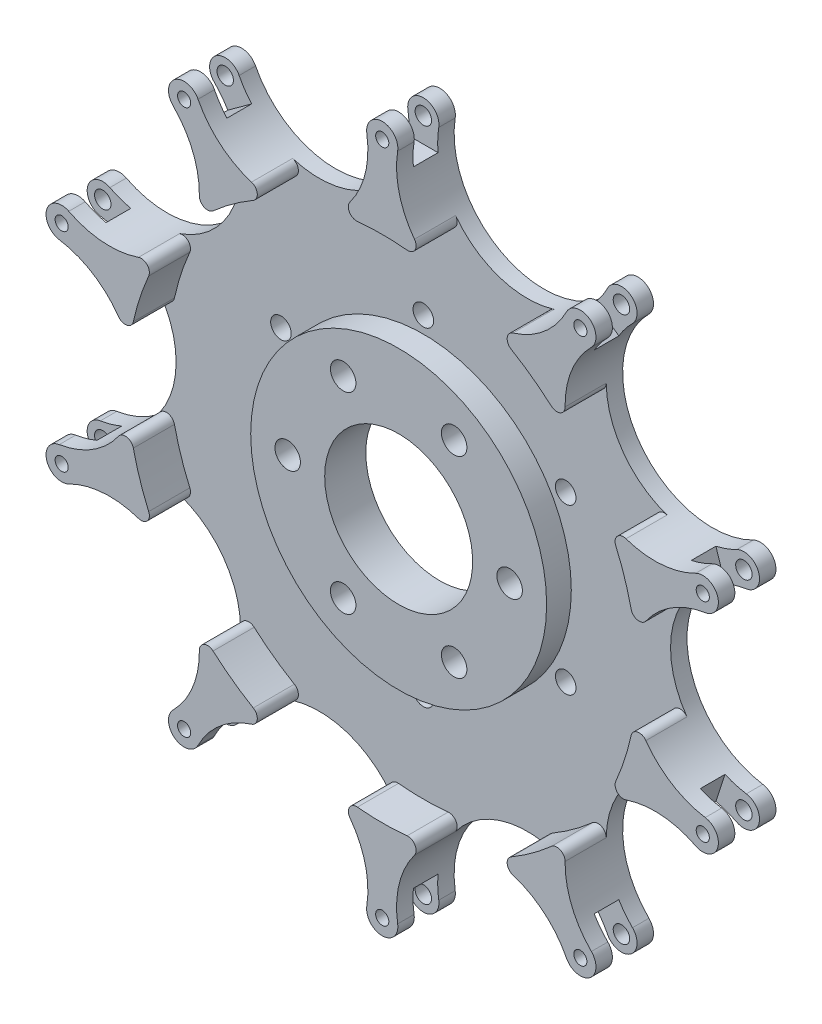
SolidWorks part; units mm, degrees
material "6061 合金"
ref_plane "前视基准面" through (0, 0, 0) normal (0, 0, 1) x (1, 0, 0)
ref_plane "上视基准面" through (0, 0, 0) normal (0, 1, 0) x (1, 0, 0)
ref_plane "右视基准面" through (0, 0, 0) normal (1, 0, 0) x (0, 0, -1)
sketch "草图1" plane through (0, 0, 0) normal (0, 0, 1) x (1, 0, 0)
  line L0 (0, 0) -> (0, 41) construction
  circle A0 centre (0, 0) radius 30.0724 construction
  circle A1 centre (0, 0) radius 41 construction
  arc A2 (1.8766, 40.7028) -> (-1.8766, 40.7028) centre (0, 41) ccw
  circle A3 centre (0, 41) radius 1
  arc A4 (1.8766, 40.7028) -> (9.2929, 28.6005) centre (12.6697, 38.9933) ccw
  arc A5 (-1.8766, 40.7028) -> (-9.2929, 28.6005) centre (-12.6697, 38.9933) cw
  circle A6 centre (0, 41) radius 2.5 construction
  arc A7 (25.4427, 31.8262) -> (24.3291, 17.6761) centre (33.1697, 24.0992) ccw
  arc A8 (22.4063, 34.0323) -> (9.2929, 28.6005) centre (12.6697, 38.9933) cw
  arc A9 (25.4427, 31.8262) -> (22.4063, 34.0323) centre (24.0992, 33.1697) ccw
  arc A10 (39.2905, 10.7931) -> (30.0724, 0) centre (41, 0) ccw
  arc A11 (38.1307, 14.3626) -> (24.3291, 17.6761) centre (33.1697, 24.0992) cw
  arc A12 (39.2905, 10.7931) -> (38.1307, 14.3626) centre (38.9933, 12.6697) ccw
  arc A13 (38.1307, -14.3626) -> (24.3291, -17.6761) centre (33.1697, -24.0992) ccw
  arc A14 (39.2905, -10.7931) -> (30.0724, 0) centre (41, 0) cw
  arc A15 (38.1307, -14.3626) -> (39.2905, -10.7931) centre (38.9933, -12.6697) ccw
  arc A16 (22.4063, -34.0323) -> (9.2929, -28.6005) centre (12.6697, -38.9933) ccw
  arc A17 (25.4427, -31.8262) -> (24.3291, -17.6761) centre (33.1697, -24.0992) cw
  arc A18 (22.4063, -34.0323) -> (25.4427, -31.8262) centre (24.0992, -33.1697) ccw
  arc A19 (-1.8766, -40.7028) -> (-9.2929, -28.6005) centre (-12.6697, -38.9933) ccw
  arc A20 (1.8766, -40.7028) -> (9.2929, -28.6005) centre (12.6697, -38.9933) cw
  arc A21 (-1.8766, -40.7028) -> (1.8766, -40.7028) centre (0, -41) ccw
  arc A22 (-25.4427, -31.8262) -> (-24.3291, -17.6761) centre (-33.1697, -24.0992) ccw
  arc A23 (-22.4063, -34.0323) -> (-9.2929, -28.6005) centre (-12.6697, -38.9933) cw
  arc A24 (-25.4427, -31.8262) -> (-22.4063, -34.0323) centre (-24.0992, -33.1697) ccw
  arc A25 (-39.2905, -10.7931) -> (-30.0724, 0) centre (-41, 0) ccw
  arc A26 (-38.1307, -14.3626) -> (-24.3291, -17.6761) centre (-33.1697, -24.0992) cw
  arc A27 (-39.2905, -10.7931) -> (-38.1307, -14.3626) centre (-38.9933, -12.6697) ccw
  arc A28 (-38.1307, 14.3626) -> (-24.3291, 17.6761) centre (-33.1697, 24.0992) ccw
  arc A29 (-39.2905, 10.7931) -> (-30.0724, 0) centre (-41, 0) cw
  arc A30 (-38.1307, 14.3626) -> (-39.2905, 10.7931) centre (-38.9933, 12.6697) ccw
  arc A31 (-22.4063, 34.0323) -> (-9.2929, 28.6005) centre (-12.6697, 38.9933) ccw
  arc A32 (-25.4427, 31.8262) -> (-24.3291, 17.6761) centre (-33.1697, 24.0992) cw
  arc A33 (-22.4063, 34.0323) -> (-25.4427, 31.8262) centre (-24.0992, 33.1697) ccw
  circle A34 centre (-12.6697, 38.9933) radius 9 construction
  circle A36 centre (24.0992, 33.1697) radius 1
  circle A37 centre (38.9933, 12.6697) radius 1
  circle A38 centre (38.9933, -12.6697) radius 1
  circle A39 centre (24.0992, -33.1697) radius 1
  circle A40 centre (0, -41) radius 1
  circle A41 centre (-24.0992, -33.1697) radius 1
  circle A42 centre (-38.9933, -12.6697) radius 1
  circle A43 centre (-38.9933, 12.6697) radius 1
  circle A44 centre (-24.0992, 33.1697) radius 1
  point P78 (0, 0)
  point P88 (0, 0)
  point P98 (0, 0)
  point P107 (0, 0)
  dimension "D1" = 10.9276
  dimension "D2" = 82
  dimension "D3" = 3.8
  dimension "D4" = 2
  dimension "D5" = 5
  dimension "D7" = 60.1447
  dimension "D8" = 18
  dimension "D6" = 10
  dimension "D9" = 10
extrude "外型" add sketch "草图1" along normal blind 2
sketch "草图4" plane through (0, 0, 0) normal (0, 0, -1) x (-1, 0, 0)
  circle A10 centre (0, 0) radius 20 construction
  point P2 (0, 20)
  point P5 (17.3205, 10)
  point P6 (17.3205, -10)
  point P7 (0, -20)
  point P8 (-17.3205, -10)
  point P10 (0, 0)
  point P27 (-17.3205, 10)
  dimension "D2" = 6
  dimension "D1" = 40
sketch "草图6" [suppressed] plane through (0, 0, 0) normal (0, 0, -1) x (-1, 0, 0)
  arc A20 (1.8766, 40.7028) -> (22.4063, 34.0323) centre (12.6697, 38.9933) ccw
  arc A21 (1.8766, 40.7028) -> (-1.8766, 40.7028) centre (0, 41) ccw
  arc A22 (-22.4063, 34.0323) -> (-1.8766, 40.7028) centre (-12.6697, 38.9933) ccw
  arc A23 (-22.4063, 34.0323) -> (-25.4427, 31.8262) centre (-24.0992, 33.1697) ccw
  arc A24 (-38.1307, 14.3626) -> (-25.4427, 31.8262) centre (-33.1697, 24.0992) ccw
  arc A25 (-38.1307, 14.3626) -> (-39.2905, 10.7931) centre (-38.9933, 12.6697) ccw
  arc A26 (-39.2905, -10.7931) -> (-39.2905, 10.7931) centre (-41, 0) ccw
  arc A27 (-39.2905, -10.7931) -> (-38.1307, -14.3626) centre (-38.9933, -12.6697) ccw
  arc A28 (-25.4427, -31.8262) -> (-38.1307, -14.3626) centre (-33.1697, -24.0992) ccw
  arc A29 (-25.4427, -31.8262) -> (-22.4063, -34.0323) centre (-24.0992, -33.1697) ccw
  arc A30 (-1.8766, -40.7028) -> (-22.4063, -34.0323) centre (-12.6697, -38.9933) ccw
  arc A31 (-1.8766, -40.7028) -> (1.8766, -40.7028) centre (0, -41) ccw
  arc A32 (22.4063, -34.0323) -> (1.8766, -40.7028) centre (12.6697, -38.9933) ccw
  arc A33 (22.4063, -34.0323) -> (25.4427, -31.8262) centre (24.0992, -33.1697) ccw
  arc A34 (38.1307, -14.3626) -> (25.4427, -31.8262) centre (33.1697, -24.0992) ccw
  arc A35 (38.1307, -14.3626) -> (39.2905, -10.7931) centre (38.9933, -12.6697) ccw
  arc A36 (39.2905, 10.7931) -> (39.2905, -10.7931) centre (41, 0) ccw
  arc A37 (39.2905, 10.7931) -> (38.1307, 14.3626) centre (38.9933, 12.6697) ccw
  arc A38 (25.4427, 31.8262) -> (38.1307, 14.3626) centre (33.1697, 24.0992) ccw
  arc A39 (25.4427, 31.8262) -> (22.4063, 34.0323) centre (24.0992, 33.1697) ccw
  arc A40 (1.8766, 40.7028) -> (22.4063, 34.0323) centre (12.6697, 38.9933) ccw
  arc A41 (1.8766, 40.7028) -> (-1.8766, 40.7028) centre (0, 41) ccw
  arc A42 (-22.4063, 34.0323) -> (-1.8766, 40.7028) centre (-12.6697, 38.9933) ccw
  arc A43 (-22.4063, 34.0323) -> (-25.4427, 31.8262) centre (-24.0992, 33.1697) ccw
  arc A44 (-38.1307, 14.3626) -> (-25.4427, 31.8262) centre (-33.1697, 24.0992) ccw
  arc A45 (-38.1307, 14.3626) -> (-39.2905, 10.7931) centre (-38.9933, 12.6697) ccw
  arc A46 (-39.2905, -10.7931) -> (-39.2905, 10.7931) centre (-41, 0) ccw
  arc A47 (-39.2905, -10.7931) -> (-38.1307, -14.3626) centre (-38.9933, -12.6697) ccw
  arc A48 (-25.4427, -31.8262) -> (-38.1307, -14.3626) centre (-33.1697, -24.0992) ccw
  arc A49 (-25.4427, -31.8262) -> (-22.4063, -34.0323) centre (-24.0992, -33.1697) ccw
  arc A50 (-1.8766, -40.7028) -> (-22.4063, -34.0323) centre (-12.6697, -38.9933) ccw
  arc A51 (-1.8766, -40.7028) -> (1.8766, -40.7028) centre (0, -41) ccw
  arc A52 (22.4063, -34.0323) -> (1.8766, -40.7028) centre (12.6697, -38.9933) ccw
  arc A53 (22.4063, -34.0323) -> (25.4427, -31.8262) centre (24.0992, -33.1697) ccw
  arc A54 (38.1307, -14.3626) -> (25.4427, -31.8262) centre (33.1697, -24.0992) ccw
  arc A55 (38.1307, -14.3626) -> (39.2905, -10.7931) centre (38.9933, -12.6697) ccw
  arc A56 (39.2905, 10.7931) -> (39.2905, -10.7931) centre (41, 0) ccw
  arc A57 (39.2905, 10.7931) -> (38.1307, 14.3626) centre (38.9933, 12.6697) ccw
  arc A58 (25.4427, 31.8262) -> (38.1307, 14.3626) centre (33.1697, 24.0992) ccw
  arc A59 (25.4427, 31.8262) -> (22.4063, 34.0323) centre (24.0992, 33.1697) ccw
  dimension "D1" = 0
extrude "切除-拉伸3" [suppressed] cut sketch "草图6" against normal up to next
sketch "草图7" plane through (0, 0, 0) normal (0, 0, -1) x (-1, 0, 0)
  line L0 (0, 0) -> (13.5, 0) construction
  circle A0 centre (0, 0) radius 13.5 construction
  circle A1 centre (13.5, 0) radius 1.55
  circle A2 centre (6.75, -11.6913) radius 1.55
  circle A3 centre (0, 0) radius 13.5 construction
  circle A4 centre (-6.75, -11.6913) radius 1.55
  circle A5 centre (0, 0) radius 13.5 construction
  circle A6 centre (-13.5, 0) radius 1.55
  circle A7 centre (0, 0) radius 13.5 construction
  circle A8 centre (-6.75, 11.6913) radius 1.55
  circle A9 centre (0, 0) radius 13.5 construction
  circle A10 centre (6.75, 11.6913) radius 1.55
  circle A11 centre (0, 0) radius 13.5 construction
  circle A12 centre (0, 0) radius 9
  circle A13 centre (0, 13.5) radius 2 construction
  circle A14 centre (11.6913, 6.75) radius 2 construction
  circle A15 centre (11.6913, -6.75) radius 2 construction
  circle A16 centre (0, -13.5) radius 2 construction
  circle A17 centre (-11.6913, -6.75) radius 2 construction
  circle A18 centre (-11.6913, 6.75) radius 2 construction
  point P23 (0, 0)
  point P36 (0, 0)
  dimension "D1" = 27
  dimension "D2" = 3.1
  dimension "D4" = 18
  dimension "D5" = 4
  dimension "D3" = 6
  dimension "D6" = 6
hole_wizard "M3 螺纹孔1" positions "草图4" profile "草图15" tap size "M3" standard "GB" end condition through all
sketch "草图15" plane through (17.3205, 10, 0) normal (1, 0, 0) x (0, 1, 0)
  line L0 (0, 0) -> (0, 2)
  line L1 (0, 2) -> (1.25, 2)
  line L2 (1.25, 2) -> (1.25, 0)
  line L5 (1.25, 0) -> (0, 0)
  line L11 (0, -6.35) -> (0, 107.95) construction
  dimension "通孔螺纹孔钻头直径" = 2.5
  dimension "通孔螺纹孔钻头深度" = 2
cosmetic thread "孔螺纹线1" parameters "D2"=3
cosmetic thread "孔螺纹线3" parameters "D2"=3
cosmetic thread "孔螺纹线4" parameters "D2"=3
cosmetic thread "孔螺纹线5" parameters "D2"=3
cosmetic thread "孔螺纹线6" parameters "D2"=3
cosmetic thread "孔螺纹线7" parameters "D2"=3
cosmetic thread "孔螺纹线18" parameters "D2"=3
extrude "连接电机" cut sketch "草图7" against normal up to next
sketch "草图8" plane through (0, 0, 0) normal (0, 0, -1) x (-1, 0, 0)
  line L1 (-12.5, -20) -> (12.5, -20) construction
  line L2 (-12.5, -20) -> (-12.5, 20) construction
  line L3 (-12.5, 20) -> (12.5, 20) construction
  line L4 (12.5, -20) -> (12.5, 20) construction
  line L5 (-12.5, -20) -> (12.5, 20) construction
  line L6 (-12.5, 20) -> (12.5, -20) construction
  circle A0 centre (-12.5, 20) radius 3.1
  circle A1 centre (12.5, 20) radius 3.1
  circle A2 centre (12.5, -20) radius 3.1
  circle A3 centre (-12.5, -20) radius 3.1
  point P0 (0, 0)
  dimension "D3" = 6.2
  dimension "D1" = 40
  dimension "D2" = 25
extrude "预留孔位" [suppressed] cut sketch "草图8" against normal up to next
sketch "草图12" plane through (0, 0, 2) normal (0, 0, -1) x (-1, 0, 0)
  circle A0 centre (6.75, 11.6913) radius 1.55 construction
  circle A1 centre (13.5, 0) radius 1.55 construction
  circle A2 centre (6.75, -11.6913) radius 1.55 construction
  circle A3 centre (-6.75, -11.6913) radius 1.55 construction
  circle A4 centre (-13.5, 0) radius 1.55 construction
  circle A5 centre (-6.75, 11.6913) radius 1.55 construction
  circle A6 centre (0, 0) radius 9 construction
  circle A7 centre (6.75, 11.6913) radius 1.55
  circle A8 centre (13.5, 0) radius 1.55
  circle A9 centre (6.75, -11.6913) radius 1.55
  circle A10 centre (-6.75, -11.6913) radius 1.55
  circle A11 centre (-13.5, 0) radius 1.55
  circle A12 centre (-6.75, 11.6913) radius 1.55
  circle A13 centre (0, 0) radius 9
  circle A14 centre (0, 0) radius 18
  dimension "D1" = 36
extrude "凸台-拉伸1" add sketch "草图12" against normal blind 3
sketch "草图13" plane through (0, 0, 2) normal (0, 0, 1) x (1, 0, 0)
  line L0 (-1.7873, 38) -> (1.7873, 38)
  line L1 (20.8899, 31.7932) -> (23.7818, 29.6921)
  line L2 (35.5878, 13.4425) -> (36.6925, 10.0428)
  line L3 (36.6925, -10.0428) -> (35.5878, -13.4425)
  line L4 (23.7818, -29.6921) -> (20.8899, -31.7932)
  line L5 (1.7873, -38) -> (-1.7873, -38)
  line L6 (-20.8899, -31.7932) -> (-23.7818, -29.6921)
  line L7 (-35.5878, -13.4425) -> (-36.6925, -10.0428)
  line L8 (-36.6925, 10.0428) -> (-35.5878, 13.4425)
  line L9 (-23.7818, 29.6921) -> (-20.8899, 31.7932)
  circle A0 centre (0, 0) radius 30 construction
  arc A3 (-3.9202, 32.4467) -> (-1.7873, 38) centre (-12.6697, 38.9933) ccw
  arc A5 (3.022, 30.8524) -> (-3.022, 30.8524) centre (0, 0) ccw
  arc A6 (-3.022, 30.8524) -> (-3.9202, 32.4467) centre (-3.1195, 31.8476) cw
  arc A7 (3.9202, 32.4467) -> (3.022, 30.8524) centre (3.1195, 31.8476) cw
  circle A10 centre (0, 34.5) radius 1.5 construction
  arc A11 (-22.4063, 34.0323) -> (-1.8766, 40.7028) centre (-12.6697, 38.9933) ccw construction
  circle A20 centre (0, 41) radius 1 construction
  arc A21 (-22.4063, 34.0323) -> (-1.8766, 40.7028) centre (-12.6697, 38.9933) ccw
  arc A22 (-22.4063, 34.0323) -> (-25.4427, 31.8262) centre (-24.0992, 33.1697) ccw
  arc A23 (-38.1307, 14.3626) -> (-25.4427, 31.8262) centre (-33.1697, 24.0992) ccw
  arc A24 (-38.1307, 14.3626) -> (-39.2905, 10.7931) centre (-38.9933, 12.6697) ccw
  arc A25 (-39.2905, -10.7931) -> (-39.2905, 10.7931) centre (-41, 0) ccw
  arc A26 (-39.2905, -10.7931) -> (-38.1307, -14.3626) centre (-38.9933, -12.6697) ccw
  arc A27 (-25.4427, -31.8262) -> (-38.1307, -14.3626) centre (-33.1697, -24.0992) ccw
  arc A28 (-25.4427, -31.8262) -> (-22.4063, -34.0323) centre (-24.0992, -33.1697) ccw
  arc A29 (-1.8766, -40.7028) -> (-22.4063, -34.0323) centre (-12.6697, -38.9933) ccw
  arc A30 (-1.8766, -40.7028) -> (1.8766, -40.7028) centre (0, -41) ccw
  arc A31 (22.4063, -34.0323) -> (1.8766, -40.7028) centre (12.6697, -38.9933) ccw
  arc A32 (22.4063, -34.0323) -> (25.4427, -31.8262) centre (24.0992, -33.1697) ccw
  arc A33 (38.1307, -14.3626) -> (25.4427, -31.8262) centre (33.1697, -24.0992) ccw
  arc A34 (38.1307, -14.3626) -> (39.2905, -10.7931) centre (38.9933, -12.6697) ccw
  arc A35 (39.2905, 10.7931) -> (39.2905, -10.7931) centre (41, 0) ccw
  arc A36 (39.2905, 10.7931) -> (38.1307, 14.3626) centre (38.9933, 12.6697) ccw
  arc A37 (25.4427, 31.8262) -> (38.1307, 14.3626) centre (33.1697, 24.0992) ccw
  arc A38 (25.4427, 31.8262) -> (22.4063, 34.0323) centre (24.0992, 33.1697) ccw
  arc A39 (1.8766, 40.7028) -> (22.4063, 34.0323) centre (12.6697, 38.9933) ccw
  arc A40 (1.8766, 40.7028) -> (-1.8766, 40.7028) centre (0, 41) ccw
  arc A59 (1.7873, 38) -> (3.9202, 32.4467) centre (12.6697, 38.9933) ccw
  arc A68 (23.7818, 29.6921) -> (22.2431, 23.9457) centre (33.1697, 24.0992) ccw
  arc A77 (22.2431, 23.9457) -> (20.5794, 23.1838) centre (21.2432, 23.9317) cw
  arc A80 (20.5794, 23.1838) -> (15.6897, 26.7364) centre (0, 0) ccw
  arc A81 (15.6897, 26.7364) -> (15.9002, 28.5541) centre (16.1958, 27.5988) cw
  arc A82 (15.9002, 28.5541) -> (20.8899, 31.7932) centre (12.6697, 38.9933) ccw
  arc A83 (36.6925, 10.0428) -> (32.07, 6.2983) centre (41, 0) ccw
  arc A84 (32.07, 6.2983) -> (30.2762, 6.6598) centre (31.2528, 6.8747) cw
  arc A85 (30.2762, 6.6598) -> (28.4085, 12.408) centre (0, 0) ccw
  arc A86 (28.4085, 12.408) -> (29.6472, 13.7549) centre (29.3249, 12.8082) cw
  arc A87 (29.6472, 13.7549) -> (35.5878, 13.4425) centre (33.1697, 24.0992) ccw
  arc A88 (35.5878, -13.4425) -> (29.6472, -13.7549) centre (33.1697, -24.0992) ccw
  arc A89 (29.6472, -13.7549) -> (28.4085, -12.408) centre (29.3249, -12.8082) cw
  arc A90 (28.4085, -12.408) -> (30.2762, -6.6598) centre (0, 0) ccw
  arc A91 (30.2762, -6.6598) -> (32.07, -6.2983) centre (31.2528, -6.8747) cw
  arc A92 (32.07, -6.2983) -> (36.6925, -10.0428) centre (41, 0) ccw
  arc A93 (20.8899, -31.7932) -> (15.9002, -28.5541) centre (12.6697, -38.9933) ccw
  arc A94 (15.9002, -28.5541) -> (15.6897, -26.7364) centre (16.1958, -27.5988) cw
  arc A95 (15.6897, -26.7364) -> (20.5794, -23.1838) centre (0, 0) ccw
  arc A96 (20.5794, -23.1838) -> (22.2431, -23.9457) centre (21.2432, -23.9317) cw
  arc A97 (22.2431, -23.9457) -> (23.7818, -29.6921) centre (33.1697, -24.0992) ccw
  arc A98 (-1.7873, -38) -> (-3.9202, -32.4467) centre (-12.6697, -38.9933) ccw
  arc A99 (-3.9202, -32.4467) -> (-3.022, -30.8524) centre (-3.1195, -31.8476) cw
  arc A100 (-3.022, -30.8524) -> (3.022, -30.8524) centre (0, 0) ccw
  arc A101 (3.022, -30.8524) -> (3.9202, -32.4467) centre (3.1195, -31.8476) cw
  arc A102 (3.9202, -32.4467) -> (1.7873, -38) centre (12.6697, -38.9933) ccw
  arc A103 (-23.7818, -29.6921) -> (-22.2431, -23.9457) centre (-33.1697, -24.0992) ccw
  arc A104 (-22.2431, -23.9457) -> (-20.5794, -23.1838) centre (-21.2432, -23.9317) cw
  arc A105 (-20.5794, -23.1838) -> (-15.6897, -26.7364) centre (0, 0) ccw
  arc A106 (-15.6897, -26.7364) -> (-15.9002, -28.5541) centre (-16.1958, -27.5988) cw
  arc A107 (-15.9002, -28.5541) -> (-20.8899, -31.7932) centre (-12.6697, -38.9933) ccw
  arc A108 (-36.6925, -10.0428) -> (-32.07, -6.2983) centre (-41, 0) ccw
  arc A109 (-32.07, -6.2983) -> (-30.2762, -6.6598) centre (-31.2528, -6.8747) cw
  arc A110 (-30.2762, -6.6598) -> (-28.4085, -12.408) centre (0, 0) ccw
  arc A111 (-28.4085, -12.408) -> (-29.6472, -13.7549) centre (-29.3249, -12.8082) cw
  arc A112 (-29.6472, -13.7549) -> (-35.5878, -13.4425) centre (-33.1697, -24.0992) ccw
  arc A113 (-35.5878, 13.4425) -> (-29.6472, 13.7549) centre (-33.1697, 24.0992) ccw
  arc A114 (-29.6472, 13.7549) -> (-28.4085, 12.408) centre (-29.3249, 12.8082) cw
  arc A115 (-28.4085, 12.408) -> (-30.2762, 6.6598) centre (0, 0) ccw
  arc A116 (-30.2762, 6.6598) -> (-32.07, 6.2983) centre (-31.2528, 6.8747) cw
  arc A117 (-32.07, 6.2983) -> (-36.6925, 10.0428) centre (-41, 0) ccw
  arc A118 (-20.8899, 31.7932) -> (-15.9002, 28.5541) centre (-12.6697, 38.9933) ccw
  arc A119 (-15.9002, 28.5541) -> (-15.6897, 26.7364) centre (-16.1958, 27.5988) cw
  arc A120 (-15.6897, 26.7364) -> (-20.5794, 23.1838) centre (0, 0) ccw
  arc A121 (-20.5794, 23.1838) -> (-22.2431, 23.9457) centre (-21.2432, 23.9317) cw
  arc A122 (-22.2431, 23.9457) -> (-23.7818, 29.6921) centre (-33.1697, 24.0992) ccw
  point P27 (-5.8696, 30.4392)
  point P36 (5.8696, 30.4392)
  point P152 (0, 0)
  point P217 (0, 0)
  dimension "D1" = 60
  dimension "D3" = 3
  dimension "D4" = 10
  dimension "D5" = 1
  dimension "D6" = 1
  dimension "D7" = 3
  dimension "D8" = 6.5
  dimension "D2" = 0
extrude "凸台-拉伸2" add sketch "草图13" along normal blind 3
sketch "草图14" plane through (0, 0, 5) normal (0, 0, 1) x (1, 0, 0)
  arc A0 (1.8766, 40.7028) -> (1.7873, 38) centre (12.6697, 38.9933) ccw construction
  arc A1 (1.8766, 40.7028) -> (-1.8766, 40.7028) centre (0, 41) ccw construction
  arc A2 (-1.7873, 38) -> (-1.8766, 40.7028) centre (-12.6697, 38.9933) ccw construction
  arc A3 (-3.9202, 32.4467) -> (-3.022, 30.8524) centre (-3.1195, 31.8476) ccw construction
  arc A4 (3.022, 30.8524) -> (-3.022, 30.8524) centre (0, 0) ccw construction
  arc A5 (3.022, 30.8524) -> (3.9202, 32.4467) centre (3.1195, 31.8476) ccw construction
  arc A6 (1.7873, 38) -> (3.9202, 32.4467) centre (12.6697, 38.9933) ccw construction
  arc A7 (-3.9202, 32.4467) -> (-1.7873, 38) centre (-12.6697, 38.9933) ccw construction
  arc A8 (1.8766, 40.7028) -> (1.7873, 38) centre (12.6697, 38.9933) ccw
  arc A9 (1.8766, 40.7028) -> (-1.8766, 40.7028) centre (0, 41) ccw
  arc A10 (-1.7873, 38) -> (-1.8766, 40.7028) centre (-12.6697, 38.9933) ccw
  arc A11 (-3.9202, 32.4467) -> (-3.022, 30.8524) centre (-3.1195, 31.8476) ccw
  arc A12 (3.022, 30.8524) -> (-3.022, 30.8524) centre (0, 0) ccw
  arc A13 (3.022, 30.8524) -> (3.9202, 32.4467) centre (3.1195, 31.8476) ccw
  arc A14 (1.7873, 38) -> (3.9202, 32.4467) centre (12.6697, 38.9933) ccw
  arc A15 (-3.9202, 32.4467) -> (-1.7873, 38) centre (-12.6697, 38.9933) ccw
  arc A18 (20.8899, 31.7932) -> (22.4063, 34.0323) centre (12.6697, 38.9933) ccw
  arc A19 (25.4427, 31.8262) -> (22.4063, 34.0323) centre (24.0992, 33.1697) ccw
  arc A20 (25.4427, 31.8262) -> (23.7818, 29.6921) centre (33.1697, 24.0992) ccw
  arc A21 (23.7818, 29.6921) -> (22.2431, 23.9457) centre (33.1697, 24.0992) ccw
  arc A22 (20.5794, 23.1838) -> (22.2431, 23.9457) centre (21.2432, 23.9317) ccw
  arc A23 (20.5794, 23.1838) -> (15.6897, 26.7364) centre (0, 0) ccw
  arc A24 (15.9002, 28.5541) -> (15.6897, 26.7364) centre (16.1958, 27.5988) ccw
  arc A25 (15.9002, 28.5541) -> (20.8899, 31.7932) centre (12.6697, 38.9933) ccw
  arc A27 (35.5878, 13.4425) -> (38.1307, 14.3626) centre (33.1697, 24.0992) ccw
  arc A28 (39.2905, 10.7931) -> (38.1307, 14.3626) centre (38.9933, 12.6697) ccw
  arc A29 (39.2905, 10.7931) -> (36.6925, 10.0428) centre (41, 0) ccw
  arc A30 (36.6925, 10.0428) -> (32.07, 6.2983) centre (41, 0) ccw
  arc A31 (30.2762, 6.6598) -> (32.07, 6.2983) centre (31.2528, 6.8747) ccw
  arc A32 (30.2762, 6.6598) -> (28.4085, 12.408) centre (0, 0) ccw
  arc A33 (29.6472, 13.7549) -> (28.4085, 12.408) centre (29.3249, 12.8082) ccw
  arc A34 (29.6472, 13.7549) -> (35.5878, 13.4425) centre (33.1697, 24.0992) ccw
  arc A36 (36.6925, -10.0428) -> (39.2905, -10.7931) centre (41, 0) ccw
  arc A37 (38.1307, -14.3626) -> (39.2905, -10.7931) centre (38.9933, -12.6697) ccw
  arc A38 (38.1307, -14.3626) -> (35.5878, -13.4425) centre (33.1697, -24.0992) ccw
  arc A39 (35.5878, -13.4425) -> (29.6472, -13.7549) centre (33.1697, -24.0992) ccw
  arc A40 (28.4085, -12.408) -> (29.6472, -13.7549) centre (29.3249, -12.8082) ccw
  arc A41 (28.4085, -12.408) -> (30.2762, -6.6598) centre (0, 0) ccw
  arc A42 (32.07, -6.2983) -> (30.2762, -6.6598) centre (31.2528, -6.8747) ccw
  arc A43 (32.07, -6.2983) -> (36.6925, -10.0428) centre (41, 0) ccw
  arc A45 (23.7818, -29.6921) -> (25.4427, -31.8262) centre (33.1697, -24.0992) ccw
  arc A46 (22.4063, -34.0323) -> (25.4427, -31.8262) centre (24.0992, -33.1697) ccw
  arc A47 (22.4063, -34.0323) -> (20.8899, -31.7932) centre (12.6697, -38.9933) ccw
  arc A48 (20.8899, -31.7932) -> (15.9002, -28.5541) centre (12.6697, -38.9933) ccw
  arc A49 (15.6897, -26.7364) -> (15.9002, -28.5541) centre (16.1958, -27.5988) ccw
  arc A50 (15.6897, -26.7364) -> (20.5794, -23.1838) centre (0, 0) ccw
  arc A51 (22.2431, -23.9457) -> (20.5794, -23.1838) centre (21.2432, -23.9317) ccw
  arc A52 (22.2431, -23.9457) -> (23.7818, -29.6921) centre (33.1697, -24.0992) ccw
  arc A54 (1.7873, -38) -> (1.8766, -40.7028) centre (12.6697, -38.9933) ccw
  arc A55 (-1.8766, -40.7028) -> (1.8766, -40.7028) centre (0, -41) ccw
  arc A56 (-1.8766, -40.7028) -> (-1.7873, -38) centre (-12.6697, -38.9933) ccw
  arc A57 (-1.7873, -38) -> (-3.9202, -32.4467) centre (-12.6697, -38.9933) ccw
  arc A58 (-3.022, -30.8524) -> (-3.9202, -32.4467) centre (-3.1195, -31.8476) ccw
  arc A59 (-3.022, -30.8524) -> (3.022, -30.8524) centre (0, 0) ccw
  arc A60 (3.9202, -32.4467) -> (3.022, -30.8524) centre (3.1195, -31.8476) ccw
  arc A61 (3.9202, -32.4467) -> (1.7873, -38) centre (12.6697, -38.9933) ccw
  arc A63 (-20.8899, -31.7932) -> (-22.4063, -34.0323) centre (-12.6697, -38.9933) ccw
  arc A64 (-25.4427, -31.8262) -> (-22.4063, -34.0323) centre (-24.0992, -33.1697) ccw
  arc A65 (-25.4427, -31.8262) -> (-23.7818, -29.6921) centre (-33.1697, -24.0992) ccw
  arc A66 (-23.7818, -29.6921) -> (-22.2431, -23.9457) centre (-33.1697, -24.0992) ccw
  arc A67 (-20.5794, -23.1838) -> (-22.2431, -23.9457) centre (-21.2432, -23.9317) ccw
  arc A68 (-20.5794, -23.1838) -> (-15.6897, -26.7364) centre (0, 0) ccw
  arc A69 (-15.9002, -28.5541) -> (-15.6897, -26.7364) centre (-16.1958, -27.5988) ccw
  arc A70 (-15.9002, -28.5541) -> (-20.8899, -31.7932) centre (-12.6697, -38.9933) ccw
  arc A72 (-35.5878, -13.4425) -> (-38.1307, -14.3626) centre (-33.1697, -24.0992) ccw
  arc A73 (-39.2905, -10.7931) -> (-38.1307, -14.3626) centre (-38.9933, -12.6697) ccw
  arc A74 (-39.2905, -10.7931) -> (-36.6925, -10.0428) centre (-41, 0) ccw
  arc A75 (-36.6925, -10.0428) -> (-32.07, -6.2983) centre (-41, 0) ccw
  arc A76 (-30.2762, -6.6598) -> (-32.07, -6.2983) centre (-31.2528, -6.8747) ccw
  arc A77 (-30.2762, -6.6598) -> (-28.4085, -12.408) centre (0, 0) ccw
  arc A78 (-29.6472, -13.7549) -> (-28.4085, -12.408) centre (-29.3249, -12.8082) ccw
  arc A79 (-29.6472, -13.7549) -> (-35.5878, -13.4425) centre (-33.1697, -24.0992) ccw
  arc A81 (-36.6925, 10.0428) -> (-39.2905, 10.7931) centre (-41, 0) ccw
  arc A82 (-38.1307, 14.3626) -> (-39.2905, 10.7931) centre (-38.9933, 12.6697) ccw
  arc A83 (-38.1307, 14.3626) -> (-35.5878, 13.4425) centre (-33.1697, 24.0992) ccw
  arc A84 (-35.5878, 13.4425) -> (-29.6472, 13.7549) centre (-33.1697, 24.0992) ccw
  arc A85 (-28.4085, 12.408) -> (-29.6472, 13.7549) centre (-29.3249, 12.8082) ccw
  arc A86 (-28.4085, 12.408) -> (-30.2762, 6.6598) centre (0, 0) ccw
  arc A87 (-32.07, 6.2983) -> (-30.2762, 6.6598) centre (-31.2528, 6.8747) ccw
  arc A88 (-32.07, 6.2983) -> (-36.6925, 10.0428) centre (-41, 0) ccw
  arc A90 (-23.7818, 29.6921) -> (-25.4427, 31.8262) centre (-33.1697, 24.0992) ccw
  arc A91 (-22.4063, 34.0323) -> (-25.4427, 31.8262) centre (-24.0992, 33.1697) ccw
  arc A92 (-22.4063, 34.0323) -> (-20.8899, 31.7932) centre (-12.6697, 38.9933) ccw
  arc A93 (-20.8899, 31.7932) -> (-15.9002, 28.5541) centre (-12.6697, 38.9933) ccw
  arc A94 (-15.6897, 26.7364) -> (-15.9002, 28.5541) centre (-16.1958, 27.5988) ccw
  arc A95 (-15.6897, 26.7364) -> (-20.5794, 23.1838) centre (0, 0) ccw
  arc A96 (-22.2431, 23.9457) -> (-20.5794, 23.1838) centre (-21.2432, 23.9317) ccw
  arc A97 (-22.2431, 23.9457) -> (-23.7818, 29.6921) centre (-33.1697, 24.0992) ccw
  point P145 (0, 0)
  dimension "D1" = 10
extrude "凸台-拉伸3" add sketch "草图14" along normal blind 2
sketch "草图9" plane through (0, 0, 0) normal (0, 0, -1) x (-1, 0, 0)
  circle A0 centre (0, 0) radius 43.5
  arc A1 (1.8766, 40.7028) -> (-1.8766, 40.7028) centre (0, 41) ccw construction
  circle A2 centre (0, 41) radius 2.5
  dimension "D1" = 87
  dimension "D2" = 5
sketch "草图16" plane through (0, 0, 7) normal (0, 0, 1) x (1, 0, 0)
  point P0 (0, 41)
  point P5 (24.0992, 33.1697)
  point P6 (38.9933, 12.6697)
  point P7 (38.9933, -12.6697)
  point P8 (24.0992, -33.1697)
  point P9 (0, -41)
  point P10 (-24.0992, -33.1697)
  point P11 (-38.9933, -12.6697)
  point P12 (-38.9933, 12.6697)
  point P13 (-24.0992, 33.1697)
  point P14 (0, 0)
  dimension "D1" = 10
hole_wizard "M2 螺纹孔1" positions "草图16" profile "草图17" tap size "M2" standard "GB" end condition through all
sketch "草图17" plane through (0, 41, 7) normal (1, 0, 0) x (0, -1, 0)
  line L0 (0, 0) -> (0, 7)
  line L1 (0, 7) -> (0.8, 7)
  line L2 (0.8, 7) -> (0.8, 0)
  line L5 (0.8, 0) -> (0, 0)
  line L11 (0, -6.35) -> (0, 107.95) construction
  dimension "通孔螺纹孔钻头直径" = 1.6
  dimension "通孔螺纹孔钻头深度" = 7
cosmetic thread "孔螺纹线8" parameters "D2"=2
cosmetic thread "孔螺纹线9" parameters "D2"=2
cosmetic thread "孔螺纹线10" parameters "D2"=2
cosmetic thread "孔螺纹线11" parameters "D2"=2
cosmetic thread "孔螺纹线12" parameters "D2"=2
cosmetic thread "孔螺纹线13" parameters "D2"=2
cosmetic thread "孔螺纹线14" parameters "D2"=2
cosmetic thread "孔螺纹线15" parameters "D2"=2
cosmetic thread "孔螺纹线16" parameters "D2"=2
cosmetic thread "孔螺纹线17" parameters "D2"=2
